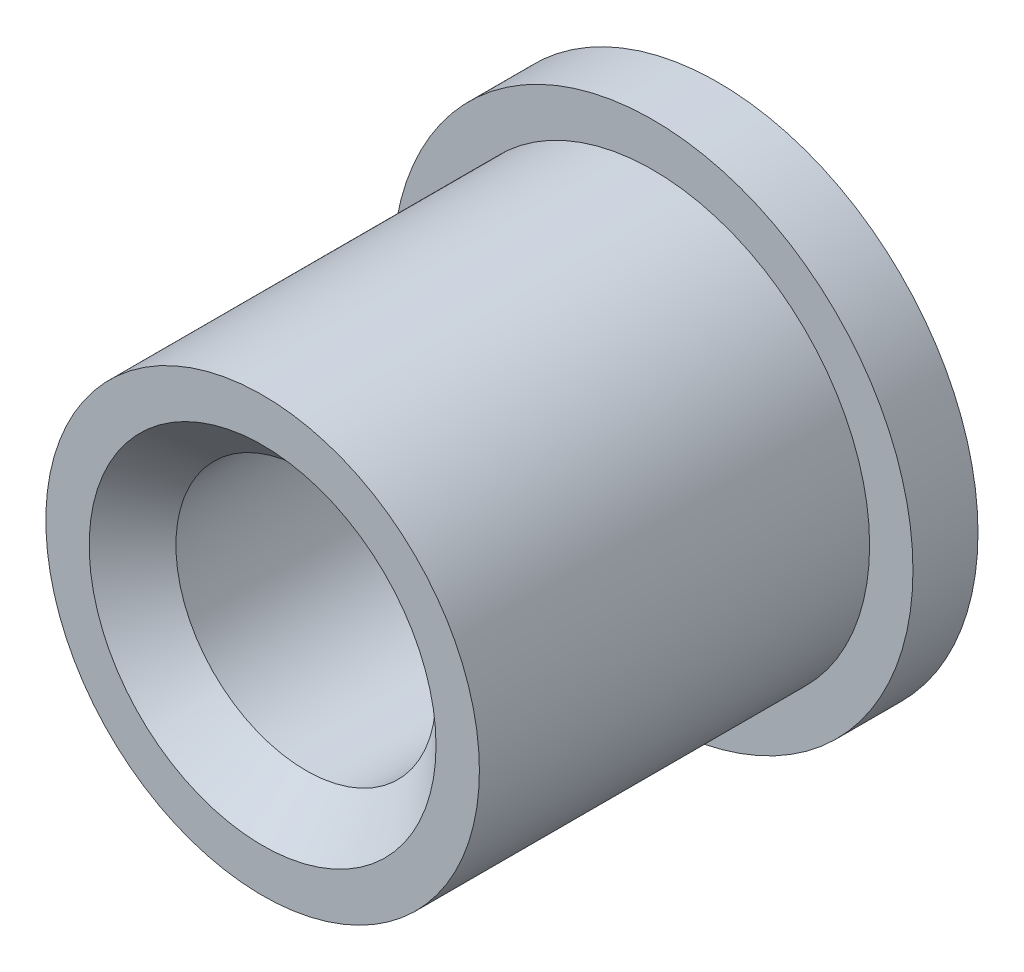
SolidWorks part; units mm, degrees
ref_plane "Front Plane" through (0, 0, 0) normal (0, 0, 1) x (1, 0, 0)
ref_plane "Top Plane" through (0, 0, 0) normal (0, 1, 0) x (1, 0, 0)
ref_plane "Right Plane" through (0, 0, 0) normal (1, 0, 0) x (0, 0, -1)
sketch "Sketch1" plane through (0, 0, 0) normal (0, 0, 1) x (1, 0, 0)
  circle A0 centre (0, 0) radius 12
  dimension "D1" = 24
extrude "Boss-Extrude1" add sketch "Sketch1" along normal blind 3
sketch "Sketch2" plane through (0, 0, 3) normal (0, 0, 1) x (1, 0, 0)
  circle A0 centre (0, 0) radius 10
  dimension "D1" = 20
extrude "Boss-Extrude2" add sketch "Sketch2" along normal blind 18
sketch "Sketch3" plane through (0, 0, 21) normal (0, 0, 1) x (1, 0, 0)
  circle A0 centre (0, 0) radius 6
  dimension "D1" = 12
extrude "Cut-Extrude1" cut sketch "Sketch3" against normal blind 26
chamfer "Chamfer1" distance 2 angle 45 1 edges at (6, 0, 21)
